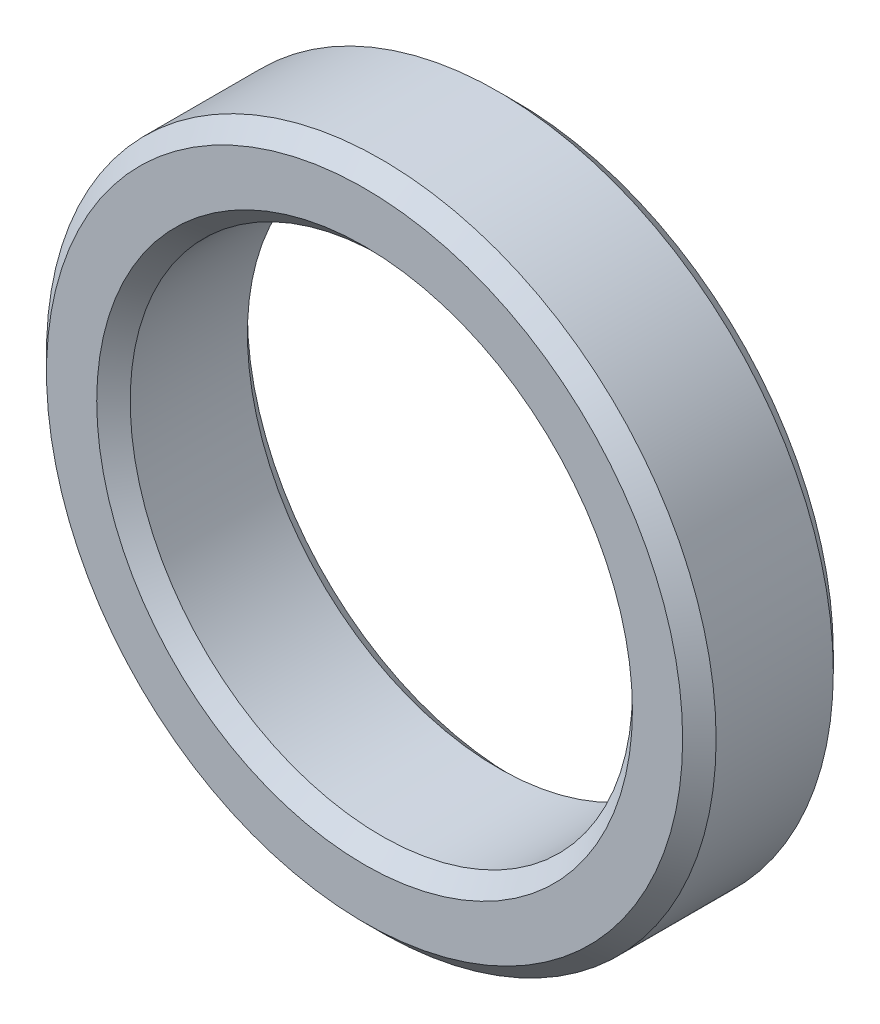
from build123d import *

# Parameters (mm, degrees)
SKETCH1_R           = 10
SKETCH1_R_2         = 7.5
BOSS_EXTRUDE1_DEPTH = 4.5
CHAMFER1_SIZE       = 0.5


with BuildPart() as part:
    # Sketch1 → Boss-Extrude1 (new body)
    with BuildSketch(Plane.XY):
        Circle(SKETCH1_R)
        Circle(SKETCH1_R_2, mode=Mode.SUBTRACT)
    extrude(amount=BOSS_EXTRUDE1_DEPTH)

    # Chamfer1
    chamfer1_edges = [part.edges().sort_by_distance(p)[0] for p in [
        (-10, 0, 0),
        (-10, 0, 4.5),
        (-7.5, 0, 0),
        (-7.5, 0, 4.5),
    ]]
    chamfer(chamfer1_edges, length=CHAMFER1_SIZE)


solid = part.part
